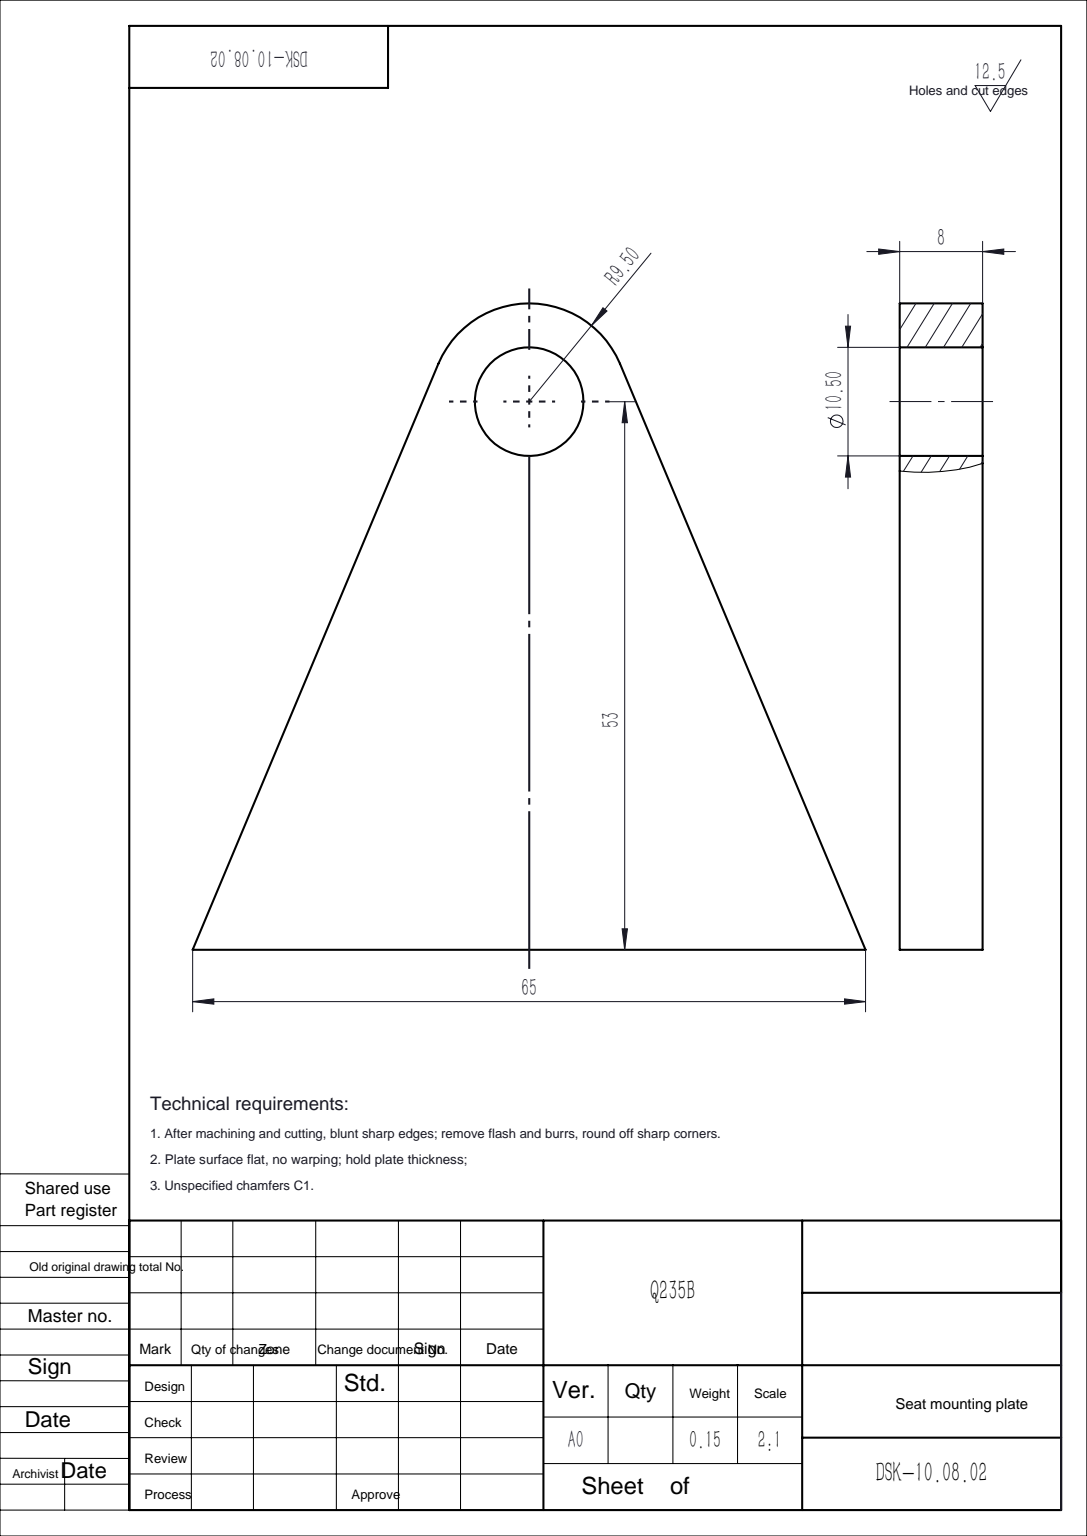
from build123d import *

# Parameters (mm, degrees)
SKETCH1_R           = 5.25
BOSS_EXTRUDE1_DEPTH = 8


with BuildPart() as part:
    # Sketch1 → Boss-Extrude1 (new body)
    with BuildSketch(Plane.XY):
        with BuildLine():
            Line((-32.5, 0), (32.5, 0))
            Line((32.5, 0), (8.762352479, 56.670310482))
            ThreePointArc((8.762352479, 56.670310482), (0, 62.5), (-8.762352479, 56.670310482))
            Line((-8.762352479, 56.670310482), (-32.5, 0))
        make_face()
        with Locations((0, 53)):
            Circle(SKETCH1_R, mode=Mode.SUBTRACT)
    extrude(amount=BOSS_EXTRUDE1_DEPTH)


solid = part.part
